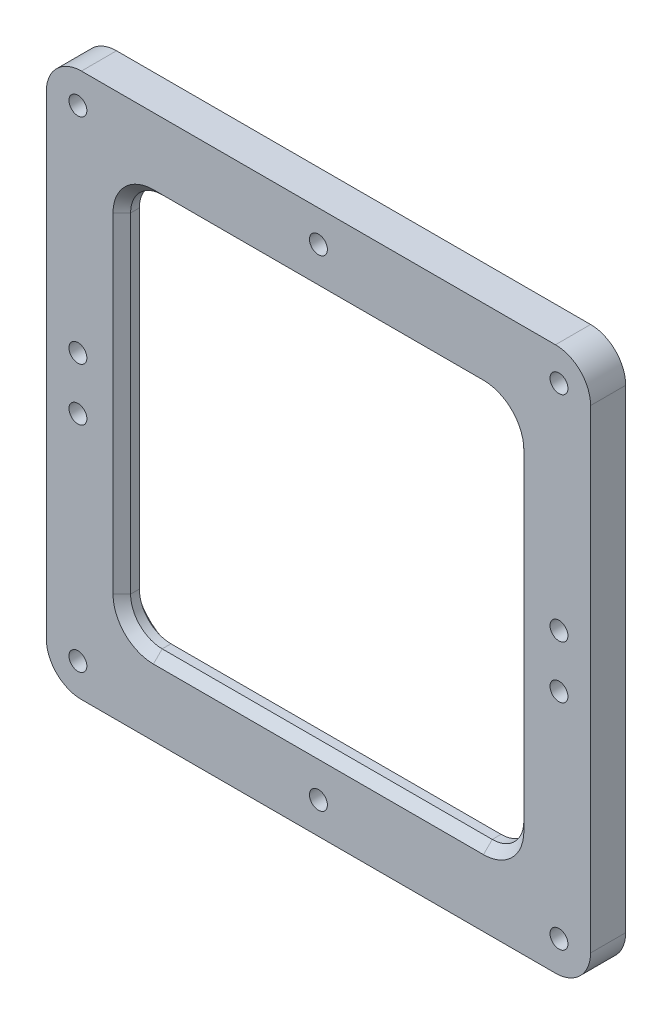
SolidWorks part; units mm, degrees
material "Q345"
ref_plane "前视基准面" through (0, 0, 0) normal (0, 0, 1) x (1, 0, 0)
ref_plane "上视基准面" through (0, 0, 0) normal (0, 1, 0) x (1, 0, 0)
ref_plane "右视基准面" through (0, 0, 0) normal (1, 0, 0) x (0, 0, -1)
sketch "草图1" plane through (0, 0, 0) normal (0, 0, 1) x (1, 0, 0)
  line L1 (-94, 112) -> (94, 112)
  line L2 (-112, 94) -> (-112, -94)
  line L3 (-94, -112) -> (94, -112)
  line L4 (112, 94) -> (112, -94)
  line L5 (-112, 112) -> (112, -112) construction
  line L6 (-112, -112) -> (112, 112) construction
  line L7 (-155, 155) -> (155, 155)
  line L8 (-155, 155) -> (-155, -155)
  line L9 (-155, -155) -> (155, -155)
  line L10 (155, 155) -> (155, -155)
  line L11 (-155, 155) -> (155, -155) construction
  line L12 (-155, -155) -> (155, 155) construction
  arc A0 (94, -112) -> (112, -94) centre (94, -94) ccw
  arc A1 (-94, -112) -> (-112, -94) centre (-94, -94) cw
  arc A2 (112, 94) -> (94, 112) centre (94, 94) ccw
  arc A3 (-112, 94) -> (-94, 112) centre (-94, 94) cw
  point P0 (0, 0)
  point P18 (0, 0)
  dimension "D3" = 18
  dimension "D1" = 224
  dimension "D2" = 224
  dimension "D4" = 310
  dimension "D5" = 310
extrude "凸台-拉伸1" add sketch "草图1" along normal blind 20
fillet "圆角1" radius 20 4 edges at (-155, -155, 10) (155, -155, 10) (-155, 155, 10) (155, 155, 10)
sketch "草图2" plane through (0, 0, 0) normal (0, 0, -1) x (-1, 0, 0)
  line L4 (0, 125.1) -> (0, 0) construction
  line L5 (0, 0) -> (0, -125.1) construction
  line L6 (125.1, 0) -> (0, 0) construction
  line L7 (0, 0) -> (-125.1, 0) construction
  line L28 (125.1, -95.1) -> (125.1, 95.1)
  line L29 (-95.1, -125.1) -> (95.1, -125.1)
  line L30 (-125.1, 95.1) -> (-125.1, -95.1)
  line L31 (95.1, 125.1) -> (-95.1, 125.1)
  arc A24 (125.1, 95.1) -> (95.1, 125.1) centre (95.1, 95.1) ccw
  arc A25 (95.1, -125.1) -> (125.1, -95.1) centre (95.1, -95.1) ccw
  arc A26 (-125.1, -95.1) -> (-95.1, -125.1) centre (-95.1, -95.1) ccw
  arc A27 (-95.1, 125.1) -> (-125.1, 95.1) centre (-95.1, 95.1) ccw
  dimension "D2" = 250.2
  dimension "D5" = 30
  dimension "D1" = 250.2
extrude "切除-拉伸1" cut sketch "草图2" against normal blind 10
sketch "草图3" plane through (0, 0, 20) normal (0, 0, -1) x (-1, 0, 0)
  line L0 (-135, 155) -> (135, 155) construction
  line L1 (-137, -137) -> (137, -137) construction
  line L2 (-137, -137) -> (-137, 137) construction
  line L3 (-137, 137) -> (137, 137) construction
  line L4 (137, -137) -> (137, 137) construction
  line L5 (-137, -137) -> (137, 137) construction
  line L6 (-137, 137) -> (137, -137) construction
  line L7 (155, 135) -> (155, -135) construction
  line L8 (0, 137) -> (0, 0) construction
  line L9 (-137, 0) -> (0, 0) construction
  line L10 (-137, 15) -> (137, 15) construction
  line L11 (-137, -15) -> (137, -15) construction
  circle A0 centre (137, 137) radius 10
  circle A1 centre (-137, 137) radius 8
  circle A2 centre (72, 137) radius 8.0759
  circle A3 centre (-72, 137) radius 8.0759
  circle A4 centre (0, 137) radius 7.5209
  circle A5 centre (137, 0) radius 12.7375
  circle A6 centre (137, 72) radius 10.7657
  circle A7 centre (137, -137) radius 10
  circle A8 centre (137, -72) radius 10.7657
  circle A9 centre (0, -137) radius 7.5209
  circle A10 centre (-72, -137) radius 8.0759
  circle A11 centre (72, -137) radius 8.0759
  circle A12 centre (-137, -72) radius 10.7657
  circle A13 centre (-137, 72) radius 10.7657
  circle A14 centre (-137, 0) radius 4.673
  circle A15 centre (-137, -137) radius 10
  point P0 (0, 0)
  point P44 (0, -15)
  point P45 (0, 15)
  dimension "D5" = 20
  dimension "D6" = 16
  dimension "D1" = 18
  dimension "D2" = 18
  dimension "D3" = 65
  dimension "D4" = 65
  dimension "D7" = 30
hole_wizard "M12 螺纹孔1" positions "3D草图1" profile "草图4" tap size "M12" standard "GB"
sketch3d "3D草图1"
  point P0 (-137, 137, 20)
  point P3 (137, 137, 20)
  point P6 (137, -137, 20)
  point P9 (-137, -137, 20)
  point P12 (0, -137, 20)
  point P21 (0, 137, 20)
  point P24 (-137, 15, 20)
  point P27 (-137, -15, 20)
  point P30 (137, 15, 20)
  point P33 (137, -15, 20)
sketch "草图4" plane through (-137, 137, 20) normal (1, 0, 0) x (0, -1, 0)
  line L0 (0, 0) -> (0, 18.0644)
  line L1 (0, 18.0644) -> (5.1, 15)
  line L2 (5.1, 15) -> (5.1, 0)
  line L5 (5.1, 0) -> (0, 0)
  line L10 (0, 18.0644) -> (-5.1, 15) construction
  line L11 (0, -6.35) -> (0, 107.95) construction
  dimension "螺纹孔钻头直径" = 10.2
  dimension "螺纹孔钻头深度" = 15
  dimension "导头角度" = 118
cosmetic thread "孔螺蚊线1" parameters "D1"=12, "D2"=12
cosmetic thread "孔螺蚊线2" parameters "D1"=12, "D2"=12
cosmetic thread "孔螺蚊线3" parameters "D1"=12, "D2"=12
cosmetic thread "孔螺蚊线4" parameters "D1"=12, "D2"=12
cosmetic thread "孔螺蚊线5" parameters "D1"=12, "D2"=12
cosmetic thread "孔螺蚊线6" parameters "D1"=12, "D2"=12
cosmetic thread "孔螺蚊线7" parameters "D1"=12, "D2"=12
cosmetic thread "孔螺蚊线8" parameters "D1"=12, "D2"=12
cosmetic thread "孔螺蚊线9" parameters "D1"=12, "D2"=12
cosmetic thread "孔螺蚊线10" parameters "D1"=12, "D2"=12
chamfer "倒角1" distance 5 angle 45 8 edges at (106.7279, -106.7279, 20) (0, -112, 20) (-106.7279, -106.7279, 20) (-112, 0, 20) (-106.7279, 106.7279, 20) (0, 112, 20) (106.7279, 106.7279, 20) (112, 0, 20)
